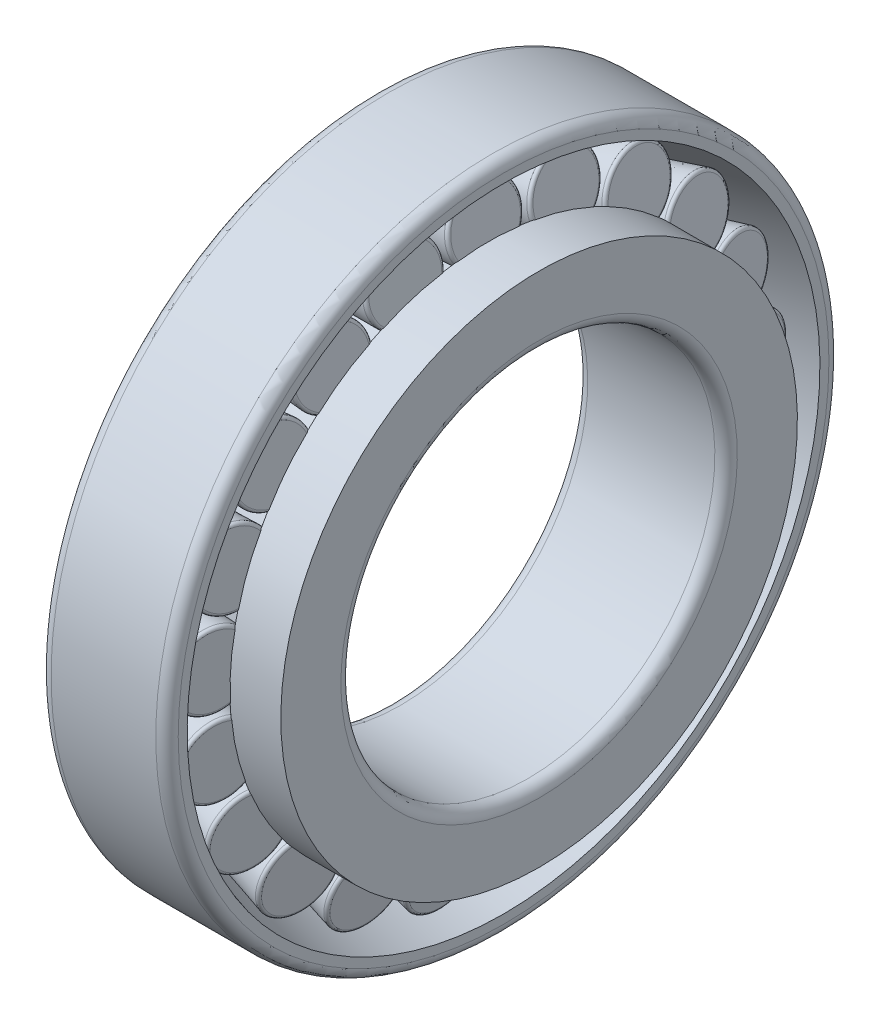
from build123d import *

# Parameters (mm, degrees)
CIRCULAR_PATTERN1_COUNT = 21


with BuildPart() as part:
    # Sketch1 → Revolve1 (revolve)
    with BuildSketch(Plane.XY, mode=Mode.PRIVATE) as revolve1_sk:
        with BuildLine():
            Line((13.25, 34.533853124), (6.436288813, 34.533853124))
            Line((6.436288813, 34.533853124), (7, 31.533853124))
            Line((7, 31.533853124), (-4.177336376, 30.429632928))
            Line((-4.177336376, 30.429632928), (-4.45919197, 31.929632928))
            Line((-4.45919197, 31.929632928), (-6.75, 31.929632928))
            Line((-6.75, 31.929632928), (-6.75, 26.5))
            ThreePointArc((-6.75, 26.5), (-6.310660172, 25.439339828), (-5.25, 25))
            Line((-5.25, 25), (11.75, 25))
            ThreePointArc((11.75, 25), (12.810660172, 25.439339828), (13.25, 26.5))
            Line((13.25, 26.5), (13.25, 34.533853124))
        make_face()
    revolve(revolve1_sk.sketch.rotate(Axis((13.25, 0, 0), (1, 0, 0)), 180), axis=Axis((13.25, 0, 0), (1, 0, 0)))

    # Sketch2 → Revolve2 (revolve)
    with BuildSketch(Plane.XY, mode=Mode.PRIVATE) as revolve2_sk:
        with BuildLine():
            Line((-4.939574193, 34.377866446), (6.096296853, 36.451547769))
            Line((6.096296853, 36.451547769), (6.943073108, 31.945111099))
            ThreePointArc((6.943073108, 31.945111099), (6.870002841, 31.631308821), (6.589277977, 31.473180127))
            Line((6.589277977, 31.473180127), (-3.82885113, 30.443962773))
            ThreePointArc((-3.82885113, 30.443962773), (-4.108109641, 30.521975183), (-4.261296192, 30.768156281))
            Line((-4.261296192, 30.768156281), (-4.939574193, 34.377866446))
        make_face()
    revolve2 = revolve(revolve2_sk.sketch.rotate(Axis((-4.939574193, 34.377866446, 0), (0.9828002416911508, 0.18467183036894297, 0)), 4.780869318), axis=Axis((-4.939574193, 34.377866446, 0), (0.9828002416911508, 0.18467183036894297, 0)))

    # Sketch3 → Revolve3 (revolve)
    with BuildSketch(Plane.XY, mode=Mode.PRIVATE) as revolve3_sk:
        with BuildLine():
            Line((-8.5, 37.539), (8.5, 42.298921142))
            Line((8.5, 42.298921142), (8.5, 43.5))
            ThreePointArc((8.5, 43.5), (8.060660172, 44.560660172), (7, 45))
            Line((7, 45), (-7, 45))
            ThreePointArc((-7, 45), (-8.060660172, 44.560660172), (-8.5, 43.5))
            Line((-8.5, 43.5), (-8.5, 37.539))
        make_face()
    revolve(revolve3_sk.sketch.rotate(Axis((13.25, 0, 0), (1, 0, 0)), 180), axis=Axis((13.25, 0, 0), (1, 0, 0)))

    # Circular-Pattern1: Revolve2 ×21 about axis
    circular_pattern1_axis = Axis((0, 0, 0), (1, 0, 0))
    for i in range(1, CIRCULAR_PATTERN1_COUNT):
        add(revolve2.rotate(circular_pattern1_axis, i * 360 / CIRCULAR_PATTERN1_COUNT))


solid = part.part
